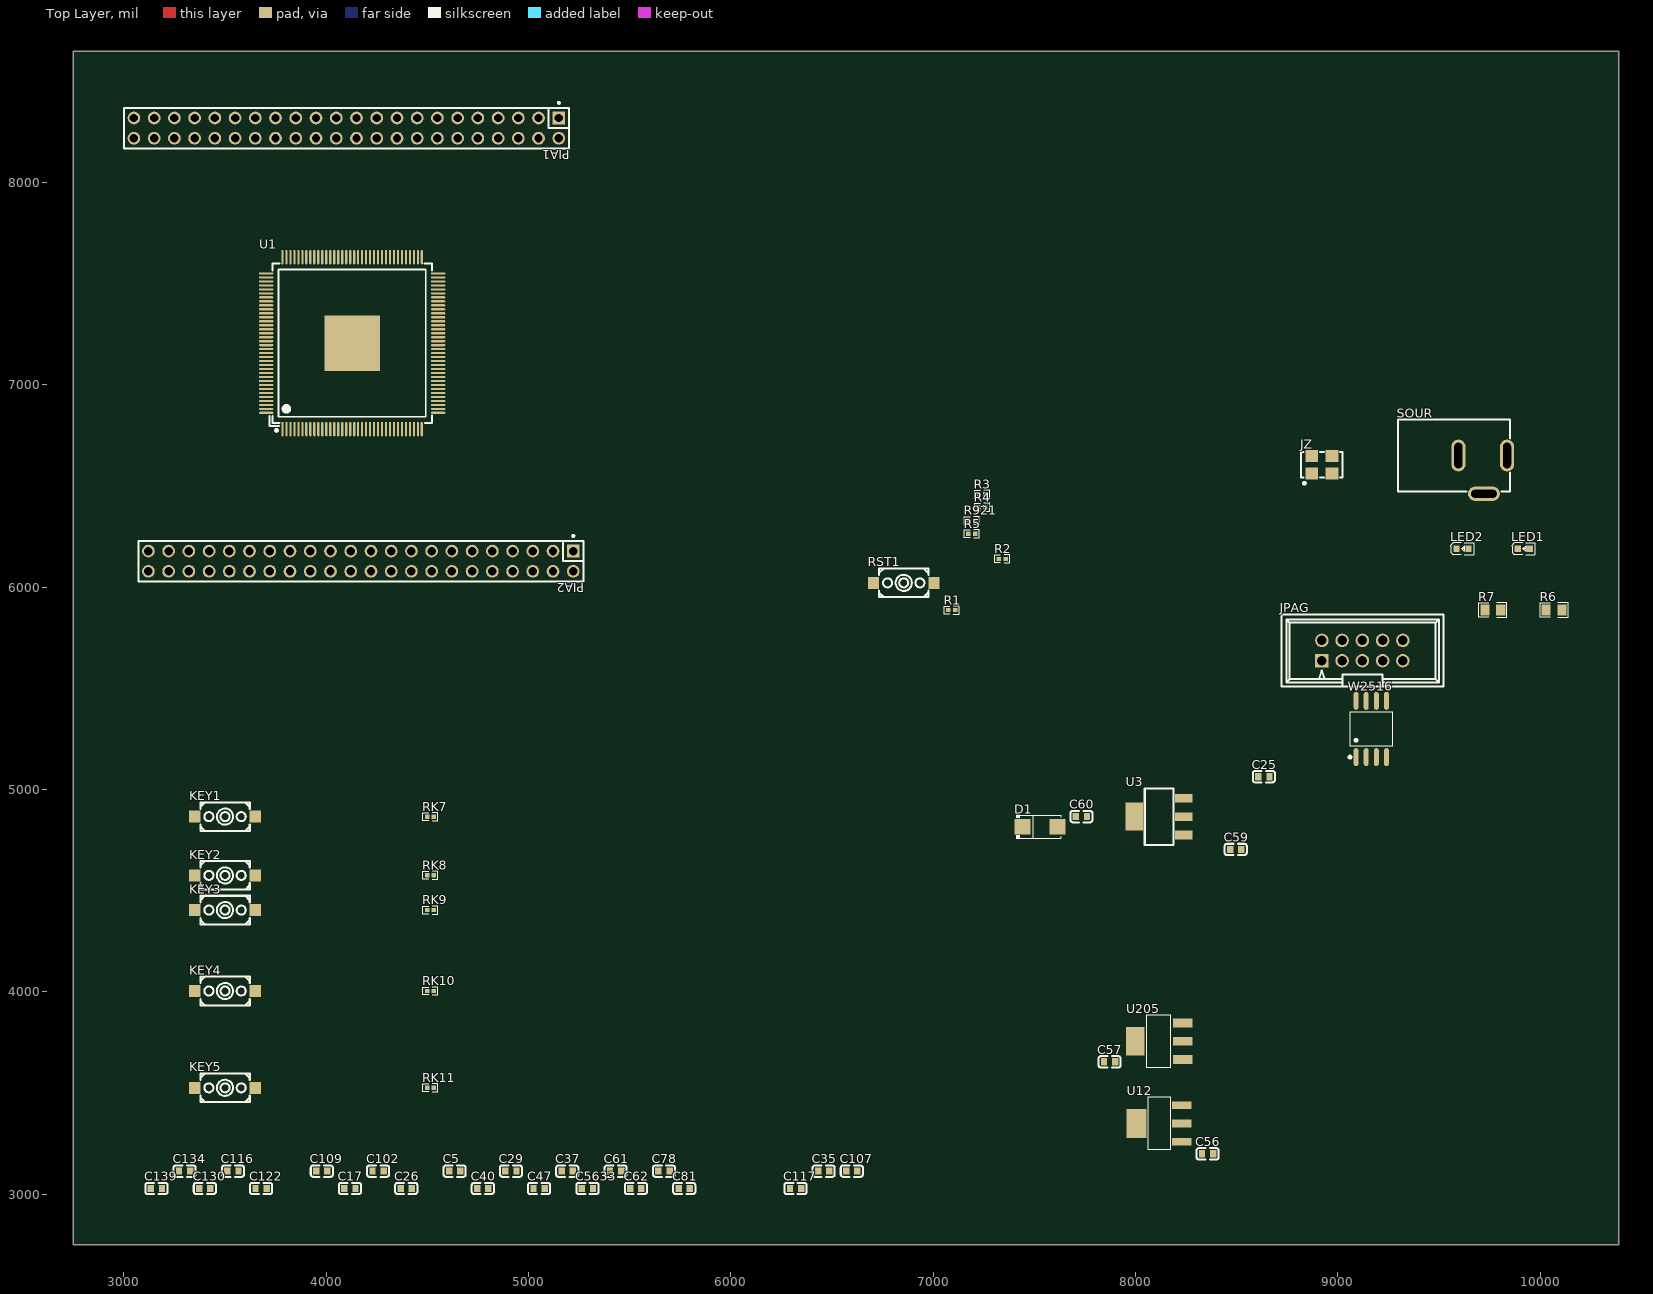
[diagram p0: Top Layer view]
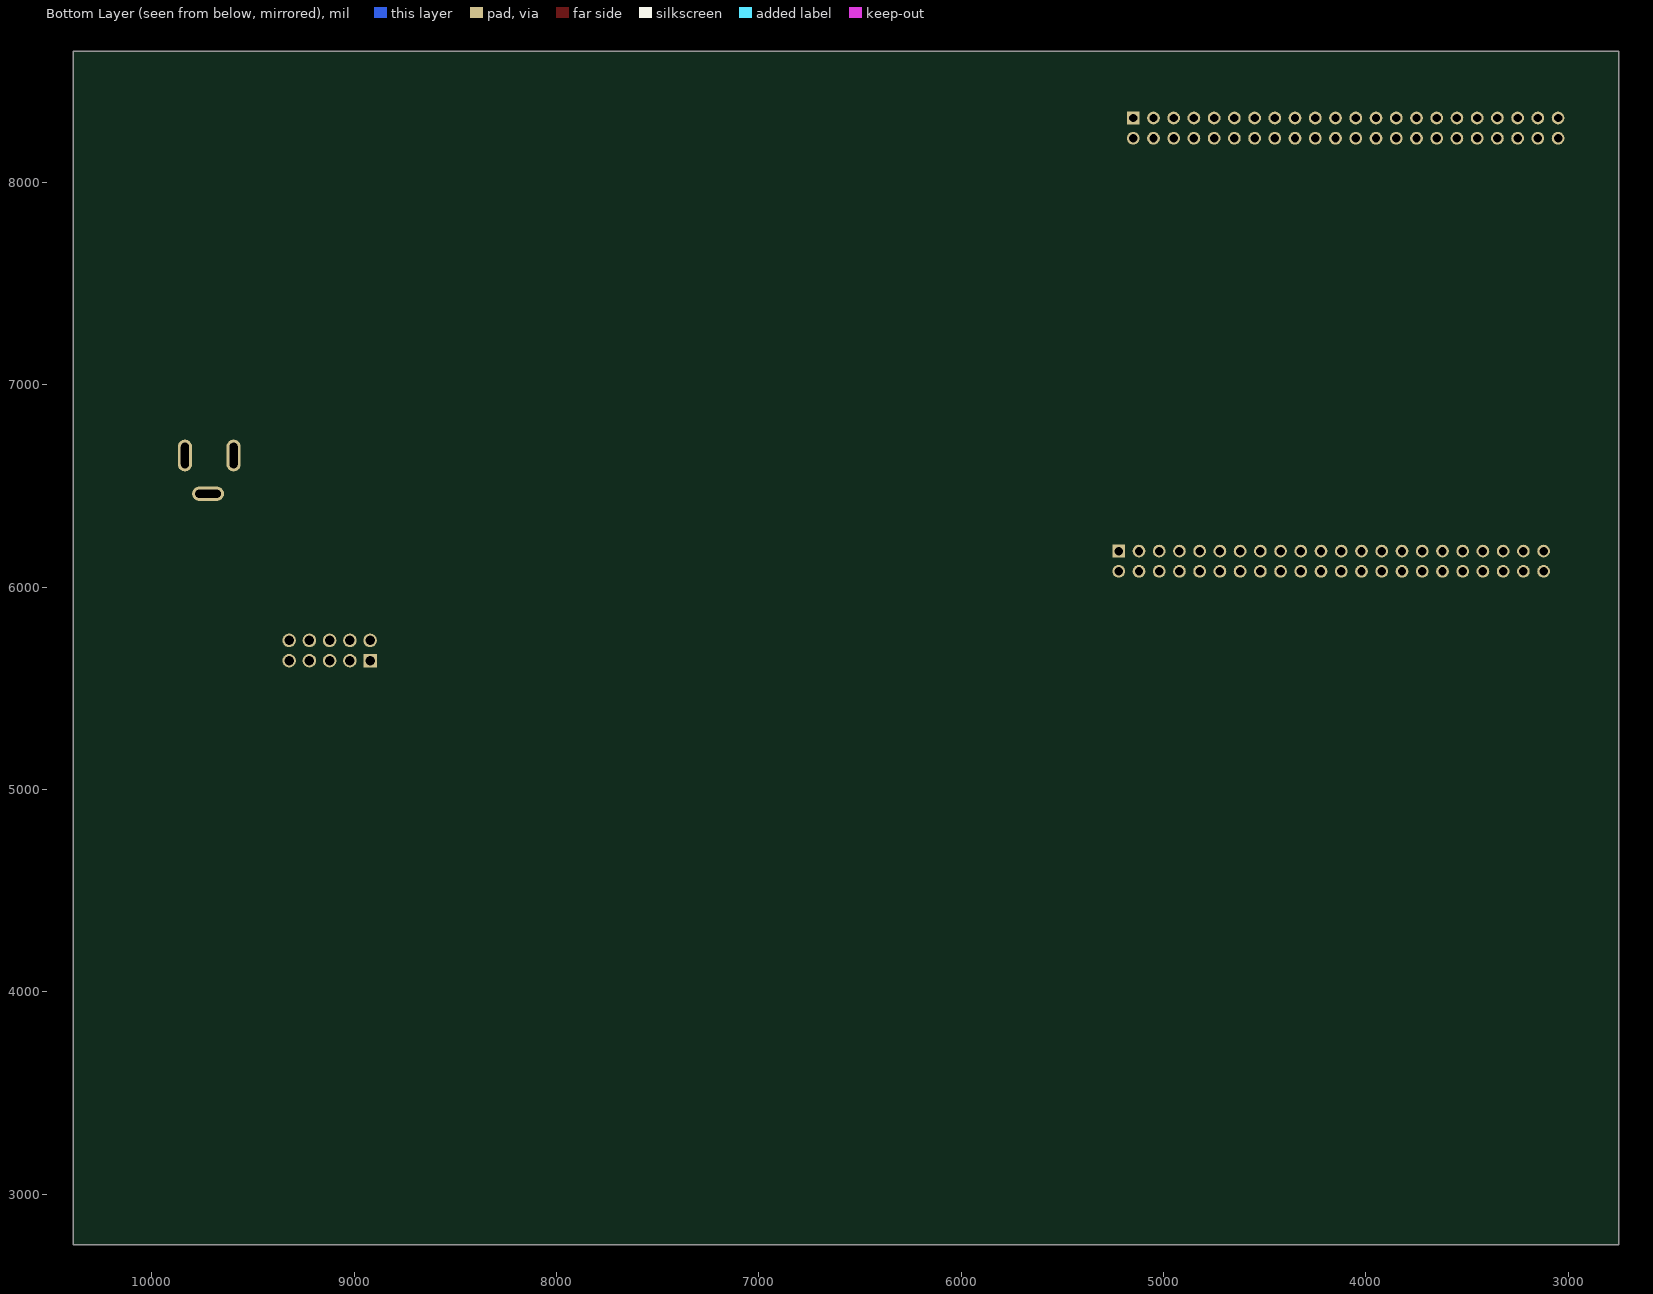
[diagram p1: Bottom Layer view, seen from below]
# Altium PCB MISC51540.pcbdoc
Units mil, origin at the board's own origin, x right, y up, seen from the top; angles counter-clockwise.
Board outline 7639.09 x 5898.92 mil, 2 copper layers (Top Layer, Bottom Layer), stack 62.206 mil thick; 59 components, 106 nets, 368 pads, 0 vias.

## Layer stack, top to bottom
Top Solder Mask Layer: solder mask 0.394, Dk 3.3
Top Layer: signal copper 1.379
Dielectric1: surface 59.449, FR4, Dk 4.5
Bottom Layer: signal copper 1.378
Bottom Solder Mask Layer: solder mask 0.394, Dk 3.3

## Board outline
10389.09,2750 2750,2750 2750,8648.92 10389.09,8648.92

## Design rules (kind name [scope] priority, off if disabled: settings)
BoardOutlineClearance copperThickness2oz_1 [All] p2 off: genericclearance=7.99 ignorepadtopadclearanceinfootprint=FALSE except(0: Arc-SplitContinuation Track-SplitContinuation SMDPad-SplitContinuation THPad-SplitContinuation Via-SplitContinuation Fill-SplitContinuation Region-SplitContinuation Poly-SplitContinuation Text-SplitContinuation Hole-SplitContinuation; 5.98: Arc-CutoutEdge SMDPad-CutoutEdge THPad-CutoutEdge Via-CutoutEdge Fill-CutoutEdge Region-CutoutEdge Text-CutoutEdge; 6.93: Hole-OutlineEdge Hole-CutoutEdge; 10: Poly-OutlineEdge Poly-CutoutEdge; 11.81: Arc-OutlineEdge Track-OutlineEdge SMDPad-OutlineEdge THPad-OutlineEdge Via-OutlineEdge Fill-OutlineEdge Region-OutlineEdge Text-OutlineEdge Track-CutoutEdge)
BoardOutlineClearance copperThickness1oz_1 [All] p4: genericclearance=4.02 ignorepadtopadclearanceinfootprint=FALSE except(0: Arc-SplitContinuation Track-SplitContinuation SMDPad-SplitContinuation THPad-SplitContinuation Via-SplitContinuation Fill-SplitContinuation Region-SplitContinuation Poly-SplitContinuation Text-SplitContinuation Hole-SplitContinuation; 6: SMDPad-CutoutEdge THPad-CutoutEdge Via-CutoutEdge Fill-CutoutEdge Region-CutoutEdge Text-CutoutEdge; 6.93: Hole-OutlineEdge Hole-CutoutEdge; 10: Poly-OutlineEdge Poly-CutoutEdge; 11.8: Arc-OutlineEdge Track-OutlineEdge SMDPad-OutlineEdge THPad-OutlineEdge Via-OutlineEdge Fill-OutlineEdge Region-OutlineEdge Text-OutlineEdge; 11.81: Arc-CutoutEdge Track-CutoutEdge)
Clearance copperThickness2oz [All] p1 off: gap=7.99 ignorepadtopadclearanceinfootprint=FALSE except(5.98: SMDPad-Track SMDPad-SMDPad THPad-Track SMDPad-THPad THPad-THPad Track-Via SMDPad-Via THPad-Via Via-Via Fill-Track Region-Track Fill-SMDPad Region-SMDPad Fill-THPad Region-THPad Fill-Via Region-Via Fill-Fill Fill-Region Region-Region Arc-Track Arc-SMDPad Arc-THPad Arc-Via Fill-Arc Region-Arc Arc-Arc Text-Track SMDPad-Text Text-THPad Text-Via Fill-Text Region-Text Arc-Text Text-Text; 6.93: Hole-Track Hole-SMDPad Hole-THPad Hole-Via Fill-Hole Region-Hole Hole-Arc Hole-Text; 10: Poly-Track Poly-SMDPad Poly-THPad Poly-Via Poly-Fill Poly-Region Poly-Poly Poly-Arc Poly-Text Poly-Hole)
Clearance copperThickness1oz [All] p3: gap=4.02 ignorepadtopadclearanceinfootprint=FALSE except(5.98: SMDPad-Track SMDPad-SMDPad THPad-Track SMDPad-THPad THPad-THPad Track-Via SMDPad-Via THPad-Via Via-Via Fill-Track Region-Track Fill-SMDPad Region-SMDPad Fill-THPad Region-THPad Fill-Via Region-Via Fill-Fill Fill-Region Region-Region; 6: Arc-Track Arc-SMDPad Arc-THPad Arc-Via Fill-Arc Region-Arc Arc-Arc Text-Track SMDPad-Text Text-THPad Text-Via Fill-Text Region-Text Arc-Text Text-Text; 6.93: Hole-Track Hole-SMDPad Hole-THPad Hole-Via Fill-Hole Region-Hole Hole-Arc Hole-Text; 10: Poly-Track Poly-SMDPad Poly-THPad Poly-Via Poly-Fill Poly-Region Poly-Poly Poly-Arc Poly-Text Poly-Hole)
DiffPairsRouting differentialPair [All] p1: maxlimit=6 minlimit=6 mostfreqgap=6 toplayer_minwidth=5 toplayer_prefwidth=10 toplayer_maxwidth=100 toplayer_mingap=6 toplayer_prefgap=6 toplayer_maxgap=6 bottomlayer_minwidth=5 bottomlayer_prefwidth=10 bottomlayer_maxwidth=100 bottomlayer_mingap=6 bottomlayer_prefgap=6 bottomlayer_maxgap=6 maxuncoupledlength=10
HoleToHoleClearance otherClearance [All] p1: gap=11.81 allowstackedmicrovias=TRUE
Length netLength [All] p1: minlimit=0 maxlimit=0
MatchedLengths netLengthTolerance [All] p1: tolerance=1000
PasteMaskExpansion pasteMaskExpansion [All] p1: expansion=0
PlaneConnect innerPlane [All] p1: planeconnectstyle=Relief reliefexpansion=20 reliefentries=4 reliefconductorwidth=10 reliefairgap=10
PolygonConnect copperRegion [All] p1: connectstyle=Relief reliefconductorwidth=10 reliefentries=4 polygonreliefangle="90 Angle" airgapwidth=10 via.connectstyle=Relief via.reliefconductorwidth=10 via.reliefentries=4 via.polygonreliefangle="90 Angle" via.airgapwidth=10
RoutingVias viaSize [All] p1: holewidth=12.01 width=24.02 viastyle="Through Hole" minholewidth=11.81 minwidth=19.68 maxholewidth=248.03 maxwidth=393.7
SolderMaskExpansion solderMaskExpansion [IsVia] p1: expansion=-1000 istentingtop=TRUE
SolderMaskExpansion solderMaskExpansion [All] p2: expansion=2 istentingtop=FALSE
Width copperThickness2oz_2 [All] p1 off: maxlimit=100 minlimit=8 preferedwidth=10
Width copperThickness1oz_2 [All] p2: maxlimit=100 minlimit=5 preferedwidth=10

## Components (designator, comment, footprint, x,y, rotation, side; value= is the part's Value field where it differs from the comment)
C5 "100nF" C0603 4635.21,3113.55 r0 top
C17 "100nF" C0603 4117.79,3027.95 r0 top
C25 "100nF" C0603 8634.89,5063.14 r0 top
C26 "100nF" C0603 4396.05,3027.95 r0 top
C29 "100nF" C0603 4913.48,3113.55 r0 top
C35 "100nF" C0603 6459.13,3113.55 r0 top
C37 "100nF" C0603 5191.74,3113.55 r0 top
C40 "100nF" C0603 4774.35,3027.95 r0 top
C47 "100nF" C0603 5052.61,3027.95 r0 top
C56 "10uF" C0603 8356.63,3199.15 r0 top
C57 "10uF" C0603 7872.28,3653.92 r0 top
C59 "10uF" C0603 8495.76,4703.84 r0 top
C60 "10uF" C0603 7733.15,4865.74 r0 top
C61 "100nF" C0603 5430.87,3113.55 r0 top
C62 "100nF" C0603 5530.87,3027.95 r0 top
C78 "100nF" C0603 5670,3113.55 r0 top
C81 "100nF" C0603 5770,3027.95 r0 top
C102 "100nF" C0603 4256.92,3113.55 r0 top
C107 "100nF" C0603 6598.26,3113.55 r0 top
C109 "100nF" C0603 3978.66,3113.55 r0 top
C116 "100nF" C0603 3539.52,3113.55 r0 top
C117 "100nF" C0603 6320,3027.95 r0 top
C122 "100nF" C0603 3678.66,3027.95 r0 top
C130 "100nF" C0603 3400.39,3027.95 r0 top
C134 "100nF" C0603 3300.39,3113.55 r0 top
C139 "100nF" C0603 3161.26,3027.95 r0 top
C5633 "100nF" C0603 5291.74,3027.95 r0 top
D1 "SMAJ5.0A-C83329" SMA_L4.3-W2.6-LS5.2-RD 7527.76,4815.74 r0 top
JPAG "MTB110-10S" IDC-TH_MTB110-10S 9121.77,5686.64 r0 top
JZ "50MHz" OSC-SMD_4P-L5.0-W3.2-BL_7CZ-XXXXX 8921.77,6606.02 r0 top
KEY1 "K2-3.6×6.1_SMD" KEY-SMD_2P-L6.2-W3.6-LS8.0 3500.39,4865.74 r0 top
KEY2 "K2-3.6×6.1_SMD" KEY-SMD_2P-L6.2-W3.6-LS8.0 3500.39,4575.34 r0 top
KEY3 "K2-3.6×6.1_SMD" KEY-SMD_2P-L6.2-W3.6-LS8.0 3500.39,4403.92 r0 top
KEY4 "K2-3.6×6.1_SMD" KEY-SMD_2P-L6.2-W3.6-LS8.0 3500.39,4003.92 r0 top
KEY5 "K2-3.6×6.1_SMD" KEY-SMD_2P-L6.2-W3.6-LS8.0 3500.39,3525.41 r0 top
LED1 "FC-1608YXK-585F08" LED0603-RD 9920.04,6189.48 r0 top
LED2 "FC-1608YXK-585F08" LED0603-RD 9616.7,6189.48 r0 top
PIA1 "X6521WV-2×22H-C30D60" HDR-TH_44P-2.54-V-M-R2-C22-S2.54 4100,8268.92 r180 top
PIA2 "X6521WV-2×22H-C30D60" HDR-TH_44P-2.54-V-M-R2-C22-S2.54 4171.54,6128.3 r180 top
R1 "10kΩ" R0402 7091.85,5886.64 r0 top
R2 "10kΩ" R0402 7341.92,6139.48 r0 top
R3 "10kΩ" R0402 7241.89,6459.37 r0 top
R4 "10kΩ" R0402 7241.89,6394.43 r0 top
R5 "10kΩ" R0402 7191.89,6264.54 r0 top
R6 "500Ω" R0805 10069.75,5886.64 r0 top
R7 "500Ω" R0805 9766.42,5886.64 r0 top
R921 "10kΩ" R0402 7191.89,6329.48 r0 top
RK7 "10kΩ" R0402 4515.63,4865.74 r0 top
RK8 "10kΩ" R0402 4515.63,4575.34 r0 top
RK9 "10kΩ" R0402 4515.63,4403.92 r0 top
RK10 "10kΩ" R0402 4515.63,4003.92 r0 top
RK11 "10kΩ" R0402 4515.63,3525.41 r0 top
RST1 "K2-3.6×6.1_SMD" KEY-SMD_2P-L6.2-W3.6-LS8.0 6854.83,6021.3 r0 top
SOUR "DC-005-2.0_C22459640" DC-IN-TH_DC-005-2.0_C22459640 9716.7,6556.02 r0 top
U1 "EP4CE6E22C8N" PQFP-144_L20.0-W20.0-P0.50-LS22.0-BL-EP 4128.65,7206.02 r0 top
U3 "TLV1117LV33DCYR" SOT-223_L6.7-W3.5-P2.30-BR 8116.99,4865.74 r0 top
U12 "TLV1117LV12DCYR" SOT-223-4_L6.5-W3.5-P2.30-LS7.0-BR 8116.99,3349.15 r0 top
U205 "TLV1117LV25DCYR" SOT-223-3_L6.5-W3.4-P2.30-LS7.0-BR 8116.99,3755.6 r0 top
W2516 "W25Q16JVSSIQ" SOIC-8_L5.3-W5.3-P1.27-LS8.0-BL 9165.84,5299.06 r0 top

## Footprints (in the part's own frame and the unit in brackets; to place one, negate y for a bottom-side part, rotate by r counter-clockwise, add the part's x,y. Pads: shape width x height; smd on the part's side, far side on the other; paste and mask are expansions set on the pad)
C0603 [mm]
  rect 0.8x0.9 smd: 1(-0.7,0) 2(0.7,0)
  silkscreen extent -1.39,-0.71 1.39,0.71
DC-IN-TH_DC-005-2.0_C22459640 [mm]
  oval 1.8x4 hole 1 slot 3.2 at 90 deg: 1(3.05,2.4) 2(-3.05,2.4)
  oval 4x1.8 hole 1 slot 3.2 at 0 deg: 3(0.15,-2.4)
  silkscreen extent -10.65,-2.1 3.45,6.9
HDR-TH_44P-2.54-V-M-R2-C22-S2.54 [mm]
  rect 1.6x1.6 hole 1.05: 1(-26.67,-1.27)
  round 1.6 hole 1.05: 2(-26.67,1.27) 3(-24.13,-1.27) 4(-24.13,1.27) 5(-21.59,-1.27) 6(-21.59,1.27) 7(-19.05,-1.27) 8(-19.05,1.27) 9(-16.51,-1.27) 10(-16.51,1.27) 11(-13.97,-1.27) 12(-13.97,1.27) 13(-11.43,-1.27) 14(-11.43,1.27) 15(-8.89,-1.27) 16(-8.89,1.27) 17(-6.35,-1.27) 18(-6.35,1.27) 19(-3.81,-1.27) 20(-3.81,1.27) 21(-1.27,-1.27) 22(-1.27,1.27) 23(1.27,-1.27) 24(1.27,1.27) 25(3.81,-1.27) 26(3.81,1.27) 27(6.35,-1.27) 28(6.35,1.27) 29(8.89,-1.27) 30(8.89,1.27) 31(11.43,-1.27) 32(11.43,1.27) 33(13.97,-1.27) 34(13.97,1.27) 35(16.51,-1.27) 36(16.51,1.27) 37(19.05,-1.27) 38(19.05,1.27) 39(21.59,-1.27) 40(21.59,1.27) 41(24.13,-1.27) 42(24.13,1.27) 43(26.67,-1.27) 44(26.67,1.27)
  silkscreen extent -27.94,-3.3 27.94,2.54
IDC-TH_MTB110-10S [mm]
  rect 1.7x1.7 hole 1.2: 1(-5.08,-1.27)
  round 1.7 hole 1.2: 2(-5.08,1.27) 3(-2.54,-1.27) 4(-2.54,1.27) 5(0,-1.27) 6(0,1.27) 7(2.54,-1.27) 8(2.54,1.27) 9(5.08,-1.27) 10(5.08,1.27)
  silkscreen extent -10.16,-4.5 10.16,4.5
KEY-SMD_2P-L6.2-W3.6-LS8.0 [mm]
  rect 1.4x1.5 smd: 1(-3.8,0) 2(3.8,0)
  silkscreen extent -3.1,-1.8 3.1,1.8
LED0603-RD [mm]
  rect 0.8x0.8 smd: 1(-0.749,0) 2(0.749,0)
  silkscreen extent -1.49,-0.75 1.39,0.76
OSC-SMD_4P-L5.0-W3.2-BL_7CZ-XXXXX [mm]
  rect 1.6x1.5 smd: 1(-1.27,-1.1) 2(1.27,-1.1) 3(1.27,1.1) 4(-1.27,1.1)
  silkscreen extent -2.6,-2.5 2.6,1.6
PQFP-144_L20.0-W20.0-P0.50-LS22.0-BL-EP [mm]
  oval 0.28x1.8 smd: 1(-8.75,-10.795) 2(-8.25,-10.795) 3(-7.75,-10.795) 4(-7.25,-10.795) 5(-6.75,-10.795) 6(-6.25,-10.795) 7(-5.75,-10.795) 8(-5.25,-10.795) 9(-4.75,-10.795) 10(-4.25,-10.795) 11(-3.75,-10.795) 12(-3.25,-10.795) 13(-2.75,-10.795) 14(-2.25,-10.795) 15(-1.75,-10.795) 16(-1.25,-10.795) 17(-0.75,-10.795) 18(-0.25,-10.795) 19(0.25,-10.795) 20(0.75,-10.795) 21(1.25,-10.795) 22(1.75,-10.795) 23(2.25,-10.795) 24(2.75,-10.795) 25(3.25,-10.795) 26(3.75,-10.795) 27(4.25,-10.795) 28(4.75,-10.795) 29(5.25,-10.795) 30(5.75,-10.795) 31(6.25,-10.795) 32(6.75,-10.795) 33(7.25,-10.795) 34(7.75,-10.795) 35(8.25,-10.795) 36(8.75,-10.795) 73(8.75,10.795) 74(8.25,10.795) 75(7.75,10.795) 76(7.25,10.795) 77(6.75,10.795) 78(6.25,10.795) 79(5.75,10.795) 80(5.25,10.795) 81(4.75,10.795) 82(4.25,10.795) 83(3.75,10.795) 84(3.25,10.795) 85(2.75,10.795) 86(2.25,10.795) 87(1.75,10.795) 88(1.25,10.795) 89(0.75,10.795) 90(0.25,10.795) 91(-0.25,10.795) 92(-0.75,10.795) 93(-1.25,10.795) 94(-1.75,10.795) 95(-2.25,10.795) 96(-2.75,10.795) 97(-3.25,10.795) 98(-3.75,10.795) 99(-4.25,10.795) 100(-4.75,10.795) 101(-5.25,10.795) 102(-5.75,10.795) 103(-6.25,10.795) 104(-6.75,10.795) 105(-7.25,10.795) 106(-7.75,10.795) 107(-8.25,10.795) 108(-8.75,10.795)
  oval 1.8x0.28 smd: 37(10.795,-8.75) 38(10.795,-8.25) 39(10.795,-7.75) 40(10.795,-7.25) 41(10.795,-6.75) 42(10.795,-6.25) 43(10.795,-5.75) 44(10.795,-5.25) 45(10.795,-4.75) 46(10.795,-4.25) 47(10.795,-3.75) 48(10.795,-3.25) 49(10.795,-2.75) 50(10.795,-2.25) 51(10.795,-1.75) 52(10.795,-1.25) 53(10.795,-0.75) 54(10.795,-0.25) 55(10.795,0.25) 56(10.795,0.75) 57(10.795,1.25) 58(10.795,1.75) 59(10.795,2.25) 60(10.795,2.75) 61(10.795,3.25) 62(10.795,3.75) 63(10.795,4.25) 64(10.795,4.75) 65(10.795,5.25) 66(10.795,5.75) 67(10.795,6.25) 68(10.795,6.75) 69(10.795,7.25) 70(10.795,7.75) 71(10.795,8.25) 72(10.795,8.75) 109(-10.795,8.75) 110(-10.795,8.25) 111(-10.795,7.75) 112(-10.795,7.25) 113(-10.795,6.75) 114(-10.795,6.25) 115(-10.795,5.75) 116(-10.795,5.25) 117(-10.795,4.75) 118(-10.795,4.25) 119(-10.795,3.75) 120(-10.795,3.25) 121(-10.795,2.75) 122(-10.795,2.25) 123(-10.795,1.75) 124(-10.795,1.25) 125(-10.795,0.75) 126(-10.795,0.25) 127(-10.795,-0.25) 128(-10.795,-0.75) 129(-10.795,-1.25) 130(-10.795,-1.75) 131(-10.795,-2.25) 132(-10.795,-2.75) 133(-10.795,-3.25) 134(-10.795,-3.75) 135(-10.795,-4.25) 136(-10.795,-4.75) 137(-10.795,-5.25) 138(-10.795,-5.75) 139(-10.795,-6.25) 140(-10.795,-6.75) 141(-10.795,-7.25) 142(-10.795,-7.75) 143(-10.795,-8.25) 144(-10.795,-8.75)
  rect 7x7 smd: 145(0,0)
  silkscreen extent -10.4,-11.1 10,10
R0402 [mm]
  rect 0.566x0.54 smd paste-100 mask+0.051: 1(-0.433,0) 2(0.433,0)
  silkscreen extent -0.94,-0.5 0.94,0.5
R0805 [mm]
  rect 1.133x1.377 smd paste-100 mask+0.051: 1(-1,0) 2(1,0)
  silkscreen extent -1.76,-0.92 1.76,0.92
SMA_L4.3-W2.6-LS5.2-RD [mm]
  rect 2x2 smd: 1(-2.2,0) 2(2.2,0)
  silkscreen extent -2.98,-1.5 2.6,1.5
SOIC-8_L5.3-W5.3-P1.27-LS8.0-BL [mm]
  oval 0.63x2.25 smd: 1(-1.905,-3.53) 2(-0.635,-3.53) 3(0.635,-3.53) 4(1.905,-3.53) 5(1.905,3.53) 6(0.635,3.53) 7(-0.635,3.53) 8(-1.905,3.53)
  silkscreen extent -2.82,-3.68 2.64,2.18
SOT-223-3_L6.5-W3.4-P2.30-LS7.0-BR [mm]
  rect 2.5x1.1 smd: 1(2.97,-2.3) 2(2.97,0) 3(2.97,2.3)
  rect 2.34x3.6 smd: 4(-2.97,0)
  silkscreen extent -1.57,-3.33 1.37,3.33
SOT-223-4_L6.5-W3.5-P2.30-LS7.0-BR [mm]
  rect 2.47x0.98 smd: 1(2.835,-2.3) 2(2.835,0) 3(2.835,2.3)
  rect 2.47x3.6 smd: 4(-2.835,0)
  silkscreen extent -1.37,-3.33 1.37,3.33
SOT-223_L6.7-W3.5-P2.30-BR [mm]
  rect 2.2x1.1 smd: 1(3.099,-2.3) 2(3.099,0) 3(3.099,2.3)
  rect 2.2x3.5 smd: 4(-3.099,0)
  silkscreen extent -1.8,-3.55 1.8,3.55

## Nets (pads, with @x,y where several pads share a name; then routed paths per layer and width w, separated by ;. In a path a pad name is that pad's centre, name@x,y a point inside that pad or via, vN(x,y) a via of type N, cw(c..) or ccw(c..) an arc to the next point about the centre after c; other vN are vias at no path point)
1.2V: C5.2 C29.2 C37.2 C56.2 C61.2 C78.2 C102.2 C109.2 C116.2 C134.2 U1.5 U1.29 U1.37 U1.45 U1.61 U1.78 U1.102 U1.109 U1.116 U1.134 U12.2 U12.4
2.5V: C35.2 C57.2 C107.2 U1.35 U1.107 U205.2 U205.4
3.3V: C17.2 C25.2 C26.2 C40.2 C47.2 C59.2 C62.2 C81.2 C117.2 C122.2 C130.2 C139.2 C5633.2 JPAG.4 JZ.4 LED1.2 LED2.2 PIA1.2 PIA2.1 R1.1 R2.1 R3.1 R4.1 R5.1 RK7.2 RK8.2 RK9.2 RK10.2 RK11.2 U1.17 U1.26 U1.40 U1.47 U1.56 U1.62 U1.81 U1.93 U1.94 U1.97 U1.117 U1.122 U1.130 U1.139 U3.2 U3.4 W2516.3 W2516.7 W2516.8
5V: C60.2 D1.1 PIA1.24 PIA2.23 SOUR.1 U3.3 U12.3 U205.3
$2N102: R2.2 U1.9
$2N244: LED2.1 R7.1
$2N245: LED1.1 R6.1
ASDO: U1.6 W2516.5
CLK: JZ.3 U1.23
CONF_DONE: R5.2 U1.92
DATA0: U1.13 W2516.2
DCLK: U1.12 W2516.6
GND: C5.1 C17.1 C25.1 C26.1 C29.1 C35.1 C37.1 C40.1 C47.1 C56.1 C57.1 C59.1 C60.1 C61.1 C62.1 C78.1 C81.1 C102.1 C107.1 C109.1 C116.1 C117.1 C122.1 C130.1 C134.1 C139.1 C5633.1 D1.2 JPAG.2 JPAG.10 JZ.2 KEY1.1 KEY2.1 KEY3.1 KEY4.1 KEY5.1 PIA1.1 PIA1.23 PIA2.2 PIA2.24 R7.2 R921.1 RST1.1 SOUR.2 SOUR.3 U1.4 U1.19 U1.22 U1.27 U1.36 U1.41 U1.48 U1.57 U1.63 U1.79 U1.82 U1.95 U1.96 U1.108 U1.118 U1.123 U1.131 U1.140 U1.145 U3.1 U12.1 U205.1 W2516.4
IO1: PIA2.29 U1.1
IO2: PIA2.30 U1.2
IO3: PIA2.27 U1.3
IO7: PIA2.28 U1.7
IO10: PIA2.25 U1.10
IO11: PIA2.26 U1.11
IO28: PIA2.21 U1.28
IO30: PIA2.22 U1.30
IO31: PIA2.19 U1.31
IO32: PIA2.20 U1.32
IO33: PIA2.17 U1.33
IO34: PIA2.18 U1.34
IO38: PIA2.15 U1.38
IO39: PIA2.16 U1.39
IO42: PIA2.13 U1.42
IO43: PIA2.14 U1.43
IO44: PIA2.11 U1.44
IO46: PIA2.12 U1.46
IO49: PIA2.9 U1.49
IO50: PIA2.10 U1.50
IO51: PIA2.7 U1.51
IO52: PIA2.8 U1.52
IO53: PIA2.5 U1.53
IO54: PIA2.6 U1.54
IO55: PIA2.3 U1.55
IO58: PIA2.4 U1.58
IO59: PIA1.3 U1.59
IO60: PIA1.4 U1.60
IO64: PIA1.5 U1.64
IO65: PIA1.6 U1.65
IO66: PIA1.7 U1.66
IO67: PIA1.8 U1.67
IO68: PIA1.9 U1.68
IO69: PIA1.10 U1.69
IO70: PIA1.11 U1.70
IO71: PIA1.12 U1.71
IO72: PIA1.13 U1.72
IO73: PIA1.14 U1.73
IO74: PIA1.15 U1.74
IO75: PIA1.16 U1.75
IO76: PIA1.17 U1.76
IO77: PIA1.18 U1.77
IO80: PIA1.19 U1.80
IO83: PIA1.20 U1.83
IO84: PIA1.21 U1.84
IO85: PIA1.22 U1.85
IO86: PIA1.25 U1.86
IO87: PIA1.26 U1.87
IO98: PIA1.27 U1.98
IO99: PIA1.28 U1.99
IO100: PIA1.29 U1.100
IO101: PIA1.30 U1.101
IO103: PIA1.31 U1.103
IO104: PIA1.32 U1.104
IO105: PIA1.33 U1.105
IO106: PIA1.34 U1.106
IO110: PIA1.35 U1.110
IO111: PIA1.36 U1.111
IO112: PIA1.37 U1.112
IO113: PIA1.38 U1.113
IO114: PIA1.39 U1.114
IO115: PIA1.40 U1.115
IO119: PIA1.41 U1.119
IO120: PIA1.42 U1.120
IO121: PIA1.43 U1.121
IO124: PIA1.44 U1.124
IO125: R6.2 U1.125
IO126: PIA2.43 U1.126
IO127: PIA2.44 U1.127
IO128: PIA2.41 U1.128
IO129: PIA2.42 U1.129
IO132: PIA2.39 U1.132
IO133: PIA2.40 U1.133
IO135: PIA2.37 U1.135
IO136: PIA2.38 U1.136
IO137: PIA2.35 U1.137
IO138: PIA2.36 U1.138
IO141: PIA2.33 U1.141
IO142: PIA2.34 U1.142
IO143: PIA2.31 U1.143
IO144: PIA2.32 U1.144
KEY1: KEY1.2 RK7.1 U1.91
KEY2: KEY2.2 RK8.1 U1.90
KEY3: KEY3.2 RK9.1 U1.89
KEY4: KEY4.2 RK10.1 U1.88
KEY5: KEY5.2 RK11.1 U1.25
NCE: R921.2 U1.21
NCONFIG: R1.2 RST1.2 U1.14
NCSO: U1.8 W2516.1
TCK: JPAG.1 U1.16
TDI: JPAG.9 R3.2 U1.15
TDO: JPAG.3 U1.20
TMS: JPAG.5 R4.2 U1.18
pads on no net: JPAG.6 JPAG.7 JPAG.8 JZ.1 U1.24